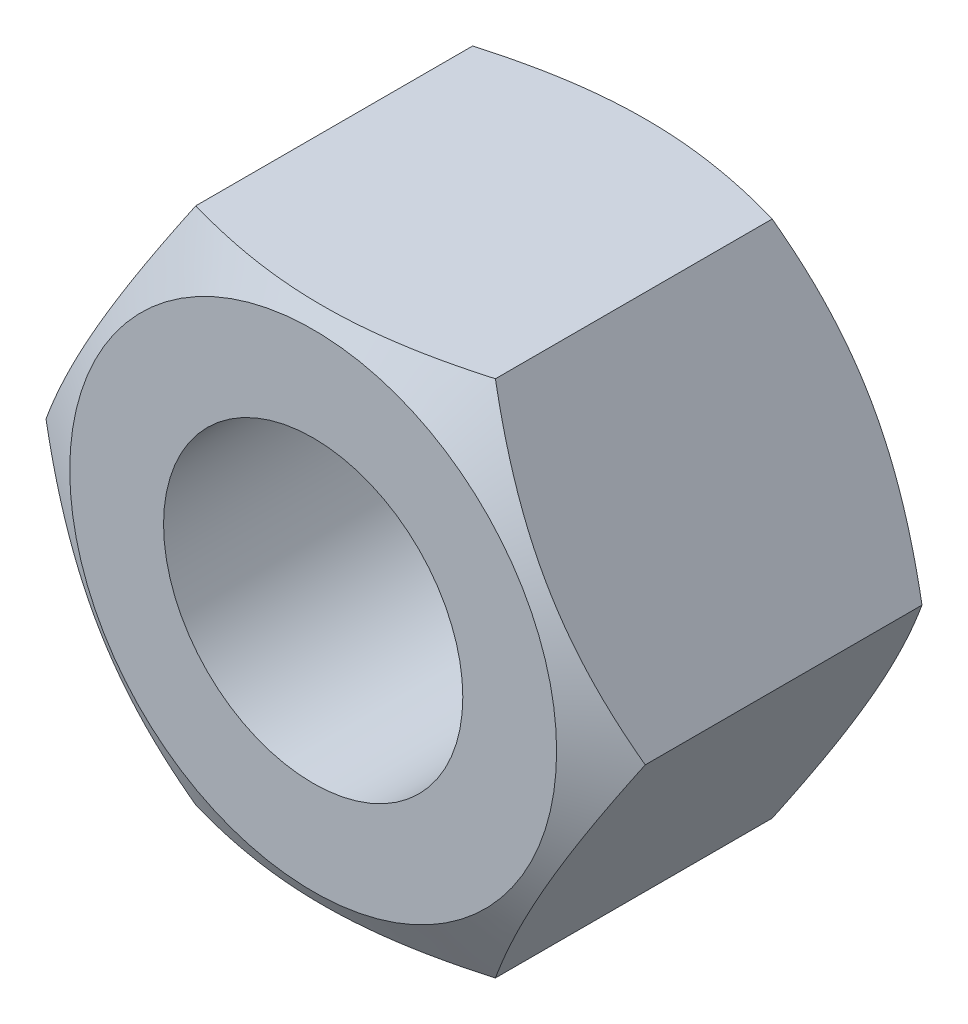
from build123d import *

# Parameters (mm, degrees)
BOSS_EXTRUDE1_DEPTH = 15.8
SKETCH3_R           = 6.92
CUT_EXTRUDE1_DEPTH  = 25.2


with BuildPart() as part:
    # Sketch1 → Boss-Extrude1 (new body)
    with BuildSketch(Plane.XY):
        Polygon((13.856406461, 0), (6.92820323, 12), (-6.92820323, 12), (-13.856406461, 0), (-6.92820323, -12), (6.92820323, -12), align=None)
    extrude(amount=BOSS_EXTRUDE1_DEPTH)

    # Sketch2 → Cut-Revolve1 (revolve, cut)
    with BuildSketch(Plane(origin=(0, 0, 0), x_dir=(1, 0, 0), z_dir=(0, 1, 0))):
        Polygon((13.856406461, -1.5), (6.92820323, 2.5), (16.856406461, 3.696152423), align=None)
        Polygon((13.856406461, -14.3), (6.92820323, -18.3), (16.856406461, -19.496152423), align=None)
    revolve(axis=Axis((0, 0, 0), (0, 0, 1)), mode=Mode.SUBTRACT)

    # Sketch3 → Cut-Extrude1 (cut, through all)
    with BuildSketch(Plane.XY):
        Circle(SKETCH3_R)
    extrude(amount=CUT_EXTRUDE1_DEPTH, mode=Mode.SUBTRACT)


solid = part.part
